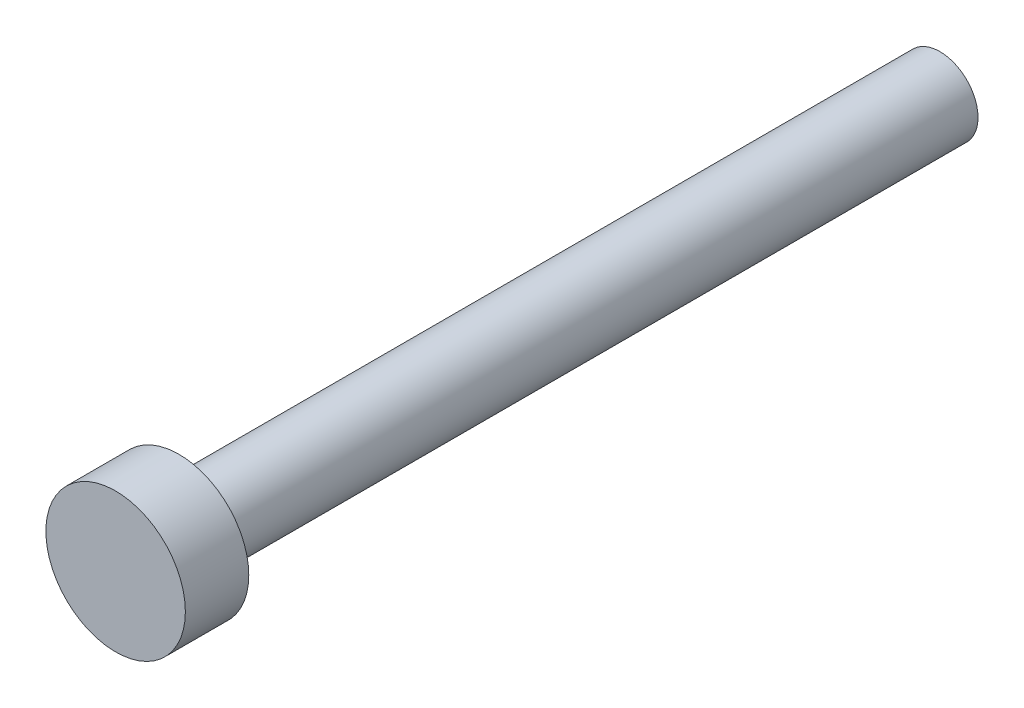
SolidWorks part; units mm, degrees
ref_plane "前视基准面" through (0, 0, 0) normal (0, 0, 1) x (1, 0, 0)
ref_plane "上视基准面" through (0, 0, 0) normal (0, 1, 0) x (1, 0, 0)
ref_plane "右视基准面" through (0, 0, 0) normal (1, 0, 0) x (0, 0, -1)
other "Configuration Table"
sketch "草图1" plane through (0, 0, 0) normal (0, 0, 1) x (1, 0, 0)
  circle A0 centre (0, 0) radius 1.5
  point P0 (0, 0)
  dimension "D1" = 3
extrude "凸台-拉伸1" add sketch "草图1" against normal blind 30
sketch "草图2" plane through (0, 0, 0) normal (0, 0, 1) x (1, 0, 0)
  circle A0 centre (0, 0) radius 2.75
  point P0 (0, 0)
  dimension "D1" = 5.5
extrude "凸台-拉伸2" add sketch "草图2" along normal blind 2.5
